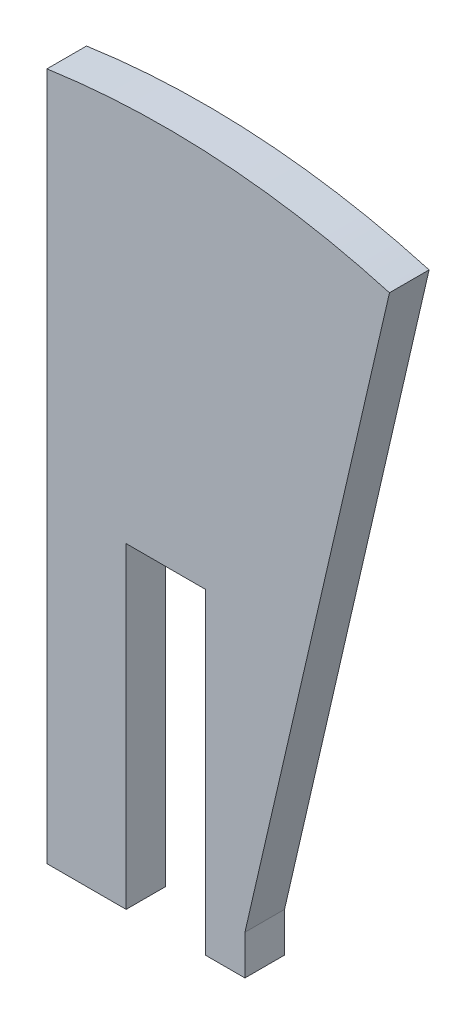
SolidWorks part; units mm, degrees
ref_plane "Front Plane" through (0, 0, 0) normal (0, 0, 1) x (1, 0, 0)
ref_plane "Top Plane" through (0, 0, 0) normal (0, 1, 0) x (1, 0, 0)
ref_plane "Right Plane" through (0, 0, 0) normal (1, 0, 0) x (0, 0, -1)
sketch "Sketch1" plane through (0, 0, 0) normal (0, 0, 1) x (1, 0, 0)
  line L0 (-30, 203.8038) -> (-30, 30)
  line L3 (20, 30) -> (20, 40)
  line L4 (20, 40) -> (56.5003, 198.1003)
  line L5 (0, 206) -> (0, 0) construction
  line L6 (20, 30) -> (-30, 30)
  arc A0 (56.5003, 198.1003) -> (-30, 203.8038) centre (0, 0) ccw
  dimension "D3" = 30
  dimension "D4" = 412
  dimension "D1" = 20
  dimension "D2" = 10
  dimension "D5" = 30
  dimension "D6" = 13
extrude "Boss-Extrude1" add sketch "Sketch1" along normal mid plane 10
sketch "Sketch2" plane through (0, 0, 5) normal (0, 0, 1) x (1, 0, 0)
  line L0 (-30, 30) -> (20, 30) construction
  line L1 (10, -50) -> (-10, -50)
  line L2 (10, -50) -> (10, 110)
  line L3 (10, 110) -> (-10, 110)
  line L4 (-10, -50) -> (-10, 110)
  line L5 (10, -50) -> (-10, 110) construction
  line L6 (10, 110) -> (-10, -50) construction
  line L7 (20, 30) -> (20, 40) construction
  point P0 (0, 30)
  dimension "D1" = 20
  dimension "D2" = 160
  dimension "D3" = 10
extrude "Cut-Extrude1" cut sketch "Sketch2" against normal blind 10
